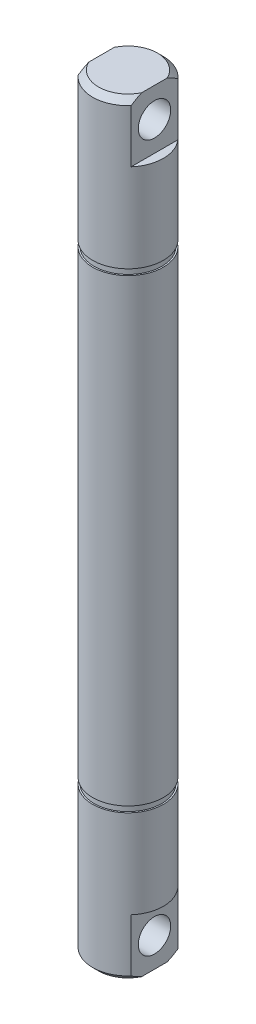
from build123d import *

# Parameters (mm, degrees)
SKETCH1_R               = 6
BOSS_EXTRUDE1_DEPTH     = 130
CUT_EXTRUDE1_DEPTH      = 131.276628756
CUT_EXTRUDE1_DEPTH_BACK = 131.276628756
SKETCH3_R               = 2.75
CHAMFER1_SIZE           = 1
SKETCH5_W               = 10
SKETCH5_H               = 20
CUT_EXTRUDE2_DEPTH      = 1.5
MIRROR2_COPY_1_SKETCH_W = 10
MIRROR2_COPY_1_SKETCH_H = 20
MIRROR2_COPY_1_DEPTH    = 1.5
SKETCH7_R               = 6
SKETCH7_R_2             = 5.75
CUT_EXTRUDE3_DEPTH      = 1


with BuildPart() as part:
    # Sketch1 → Boss-Extrude1 (new body)
    with BuildSketch(Plane(origin=(0, 0, 0), x_dir=(1, 0, 0), z_dir=(0, 1, 0))):
        with Locations(Location((0, 0, 0), (0, 0, 270))):
            Circle(SKETCH1_R)
    extrude(amount=BOSS_EXTRUDE1_DEPTH)

    # Sketch3 → Cut-Extrude1 (cut, two sides: drawn at the far end of the back side and taken through both)
    with BuildSketch(Plane(origin=(0, 0, 0), x_dir=(0, 0, -1), z_dir=(1, 0, 0)).offset(-CUT_EXTRUDE1_DEPTH_BACK)):
        with Locations((0, 125)):
            Circle(SKETCH3_R)
        with Locations((0, 5)):
            Circle(SKETCH3_R)
    extrude(amount=CUT_EXTRUDE1_DEPTH + CUT_EXTRUDE1_DEPTH_BACK, mode=Mode.SUBTRACT)

    # Chamfer1
    chamfer1_edges = [part.edges().sort_by_distance(p)[0] for p in [
        (0, 0, -6),
        (0, 130, -6),
    ]]
    chamfer(chamfer1_edges, length=CHAMFER1_SIZE)

    # Sketch5 → Cut-Extrude2 (cut)
    with BuildSketch(Plane(origin=(6, 0, 0), x_dir=(0, 0, -1), z_dir=(1, 0, 0))):
        Rectangle(SKETCH5_W, SKETCH5_H)
    cut_extrude2 = extrude(amount=-CUT_EXTRUDE2_DEPTH, mode=Mode.SUBTRACT)

    # Mirror1: Cut-Extrude2 across plane
    add(cut_extrude2.mirror(Plane(origin=(0, 0, 0), x_dir=(0, 0, 1), z_dir=(1, 0, 0))), mode=Mode.SUBTRACT)

    # Mirror2: Cut-Extrude2 across plane
    add(cut_extrude2.mirror(Plane(origin=(0, 65, 0), x_dir=(0, 0, 1), z_dir=(0, -1, 0))), mode=Mode.SUBTRACT)

    # Mirror2 copy 1 sketch → Mirror2 copy 1 (cut)
    with BuildSketch(Plane(origin=(-6, 130, 0), x_dir=(0, 0, -1), z_dir=(-1, 0, 0))):
        Rectangle(MIRROR2_COPY_1_SKETCH_W, MIRROR2_COPY_1_SKETCH_H)
    extrude(amount=-MIRROR2_COPY_1_DEPTH, mode=Mode.SUBTRACT)

    # Sketch7 → Cut-Extrude3 (cut)
    with BuildSketch(Plane(origin=(0, 104, 0), x_dir=(1, 0, 0), z_dir=(0, 1, 0))):
        with Locations(Location((0, 0, 0), (0, 0, 138.590377891))):
            Circle(SKETCH7_R)
        with Locations(Location((0, 0, 0), (0, 0, 270))):
            Circle(SKETCH7_R_2, mode=Mode.SUBTRACT)
    cut_extrude3 = extrude(amount=CUT_EXTRUDE3_DEPTH, mode=Mode.SUBTRACT)

    # Mirror3: Cut-Extrude3 across plane
    add(cut_extrude3.mirror(Plane(origin=(0, 65, 0), x_dir=(0, 0, 1), z_dir=(0, -1, 0))), mode=Mode.SUBTRACT)


solid = part.part
